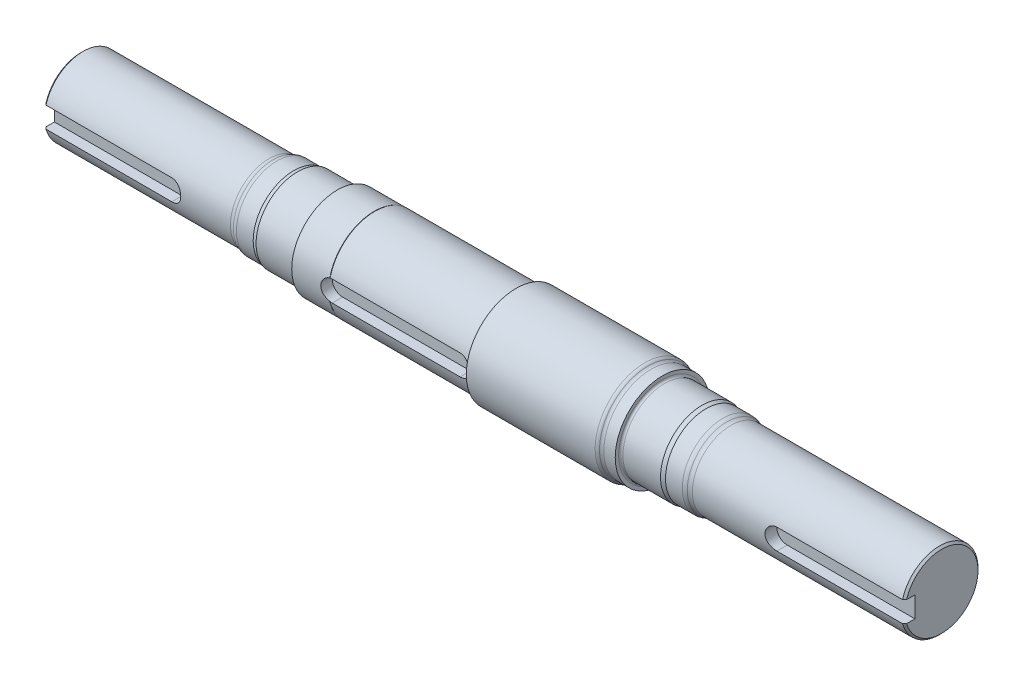
from build123d import *

# Parameters (mm, degrees)
FILLET3_R      = 3.302
FILLET4_R      = 1.524
CHAMFER1_SIZE  = 3.048
EXTRUDE1_START = 40.6766
EXTRUDE1_DEPTH = 1279.168730275
EXTRUDE2_START = 52.1601
EXTRUDE2_DEPTH = 1267.685230275


with BuildPart() as part:
    # Sketch1 → Revolve1 (revolve)
    with BuildSketch(Plane.XY, mode=Mode.PRIVATE) as revolve1_sk:
        with BuildLine():
            Line((0, 0), (0, 58.7375))
            Line((0, 58.7375), (286.967638938, 58.7375))
            ThreePointArc((286.967638938, 58.7375), (290.142638938, 59.140777876), (293.116, 60.325))
            ThreePointArc((293.116, 60.325), (296.089361062, 61.509222124), (299.264361062, 61.9125))
            Line((299.264361062, 61.9125), (324.866, 61.9125))
            Line((324.866, 61.9125), (330.861726225, 63.51905))
            Line((330.861726225, 63.51905), (391.541, 63.51905))
            Line((391.541, 63.51905), (391.541, 69.6976))
            Line((391.541, 69.6976), (447.947838412, 69.6976))
            Line((447.947838412, 69.6976), (448.564, 69.8627))
            Line((448.564, 69.8627), (664.591, 69.8627))
            Line((664.591, 69.8627), (664.591, 76.073))
            Line((664.591, 76.073), (861.363000314, 76.073))
            ThreePointArc((861.363000314, 76.073), (863.899028459, 75.544602979), (866.013, 74.04735))
            ThreePointArc((866.013, 74.04735), (868.126971541, 72.550097021), (870.662999686, 72.0217))
            Line((870.662999686, 72.0217), (888.0094, 72.0217))
            Line((888.0094, 72.0217), (888.0094, 63.51905))
            Line((888.0094, 63.51905), (948.688673775, 63.51905))
            Line((948.688673775, 63.51905), (954.6844, 61.9125))
            Line((954.6844, 61.9125), (980.286038938, 61.9125))
            ThreePointArc((980.286038938, 61.9125), (983.461038938, 61.509222124), (986.4344, 60.325))
            ThreePointArc((986.4344, 60.325), (989.407761062, 59.140777876), (992.582761062, 58.7375))
            Line((992.582761062, 58.7375), (1314.45, 58.7375))
            Line((1314.45, 58.7375), (1314.45, 0))
            Line((1314.45, 0), (0, 0))
        make_face()
    revolve(revolve1_sk.sketch.rotate(Axis((0, 0, 0), (1, 0, 0)), 90), axis=Axis((0, 0, 0), (1, 0, 0)))

    # Fillet3
    fillet3_edges = [part.edges().sort_by_distance(p)[0] for p in [
        (391.541, 0, -63.51905),
        (888.0094, 0, -63.51905),
    ]]
    fillet(fillet3_edges, radius=FILLET3_R)

    # Fillet4
    fillet4_edges = [part.edges().sort_by_distance(p)[0] for p in [
        (664.591, 0, -69.8627),
    ]]
    fillet(fillet4_edges, radius=FILLET4_R)

    # Chamfer1
    chamfer1_edges = [part.edges().sort_by_distance(p)[0] for p in [
        (0, 0, -58.7375),
        (1314.45, 0, -58.7375),
    ]]
    chamfer(chamfer1_edges, length=CHAMFER1_SIZE)

    # Sketch2 → Extrude1 (cut, through all)
    with BuildSketch(Plane.XY.offset(EXTRUDE1_START)):
        with BuildLine():
            Line((0, 15.875), (195.199, 15.875))
            ThreePointArc((195.199, 15.875), (211.074, 0), (195.199, -15.875))
            Line((195.199, -15.875), (0, -15.875))
            Line((0, -15.875), (0, 15.875))
        make_face()
        with BuildLine():
            Line((1314.45, 15.875), (1314.45, -15.875))
            Line((1314.45, -15.875), (1119.251, -15.875))
            ThreePointArc((1119.251, -15.875), (1103.376, 0), (1119.251, 15.875))
            Line((1119.251, 15.875), (1314.45, 15.875))
        make_face()
    extrude(amount=EXTRUDE1_DEPTH, mode=Mode.SUBTRACT)

    # Sketch3 → Extrude2 (cut, through all)
    with BuildSketch(Plane.XY.offset(EXTRUDE2_START)):
        with BuildLine():
            Line((451.739, -15.875), (647.101, -15.875))
            ThreePointArc((647.101, -15.875), (662.976, 0), (647.101, 15.875))
            Line((647.101, 15.875), (451.739, 15.875))
            ThreePointArc((451.739, 15.875), (435.864, 0), (451.739, -15.875))
        make_face()
    extrude(amount=EXTRUDE2_DEPTH, mode=Mode.SUBTRACT)


solid = part.part
